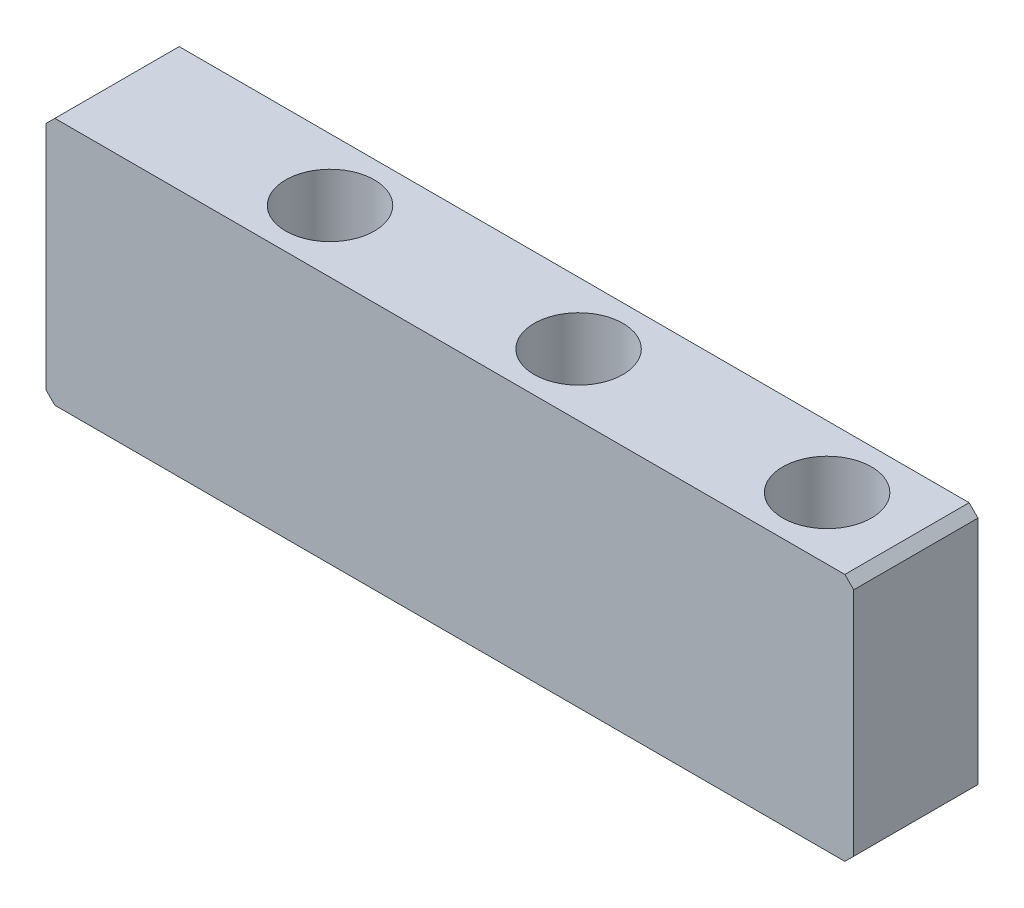
SolidWorks part; units mm, degrees
material "AL6061"
ref_plane "Front Plane" through (0, 0, 0) normal (0, 0, 1) x (1, 0, 0)
ref_plane "Top Plane" through (0, 0, 0) normal (0, 1, 0) x (1, 0, 0)
ref_plane "Right Plane" through (0, 0, 0) normal (1, 0, 0) x (0, 0, -1)
sketch "Sketch1" plane through (0, 0, 0) normal (0, 0, 1) x (1, 0, 0)
  line L1 (-45.5, -14) -> (45.5, -14)
  line L2 (-45.5, -14) -> (-45.5, 14)
  line L3 (-45.5, 14) -> (45.5, 14)
  line L4 (45.5, -14) -> (45.5, 14)
  line L5 (-45.5, -14) -> (45.5, 14) construction
  line L6 (-45.5, 14) -> (45.5, -14) construction
  point P0 (0, 0)
  dimension "D1" = 28
  dimension "D2" = 91
extrude "Boss-Extrude1" add sketch "Sketch1" along normal mid plane 14
hole_wizard "M6 Tapped Hole1" positions "Sketch2" profile "Sketch3" tap size "M6" standard "GB"
sketch "Sketch2" plane through (-45.5, 0, 0) normal (-1, 0, 0) x (0, 0, 1)
  line L0 (0, 0) -> (0, 19.6516) construction
  line L3 (0, 0) -> (11.5977, 0) construction
  line L4 (7, 14) -> (-7, 14) construction
  point P13 (0, 7)
  point P16 (0, -7)
  dimension "D1" = 7
  dimension "D2" = 14
sketch "Sketch3" plane through (-45.5, -7, 0) normal (0, 1, 0) x (0, 0, 1)
  line L0 (0, 0) -> (0, 16.5022)
  line L1 (0, 16.5022) -> (2.5, 15)
  line L2 (2.5, 15) -> (2.5, 0)
  line L5 (2.5, 0) -> (0, 0)
  line L10 (0, 16.5022) -> (-2.5, 15) construction
  line L11 (0, -6.35) -> (0, 107.95) construction
  dimension "螺纹孔钻头直径" = 5
  dimension "螺纹孔钻头深度" = 15
  dimension "导头角度" = 118
cosmetic thread "Cosmetic Thread1" parameters "D1"=12, "D2"=6
cosmetic thread "Cosmetic Thread2" parameters "D1"=12, "D2"=6
hole_wizard "Hole Size per Socket Head Cap Screw Type1" positions "Sketch4" profile "Sketch5" counterbore size "M5" standard "GB" end condition through all
sketch "Sketch4" plane through (0, 14, 0) normal (0, 1, 0) x (1, 0, 0)
  line L0 (22.3923, 0) -> (-53.4687, 0) construction
  line L1 (-45.5, -7) -> (-45.5, 7) construction
  line L2 (45.5, -7) -> (45.5, 7) construction
  point P7 (-20.5, 0)
  point P14 (35.5, 0)
  point P30 (7.5, 0)
  dimension "D1" = 25
  dimension "D2" = 10
  dimension "D3" = 56
  dimension "D4" = 28
sketch "Sketch5" plane through (7.5, 14, 0) normal (1, 0, 0) x (0, 0, 1)
  line L0 (0, 0) -> (0, 28)
  line L1 (0, 28) -> (2.75, 28)
  line L3 (2.75, 28) -> (2.75, 10)
  line L4 (2.75, 10) -> (5, 10)
  line L5 (5, 10) -> (5, 0)
  line L7 (5, 0) -> (0, 0)
  line L11 (0, -6.35) -> (0, 107.95) construction
  dimension "通孔孔直径" = 5.5
  dimension "通孔孔深度" = 28
  dimension "柱形沉头孔直径" = 10
  dimension "柱形沉头孔深度" = 10
chamfer "Chamfer1" distance 1 angle 45 4 edges at (45.5, 14, 0) (45.5, -14, 0) (-45.5, -14, 0) (-45.5, 14, 0)
